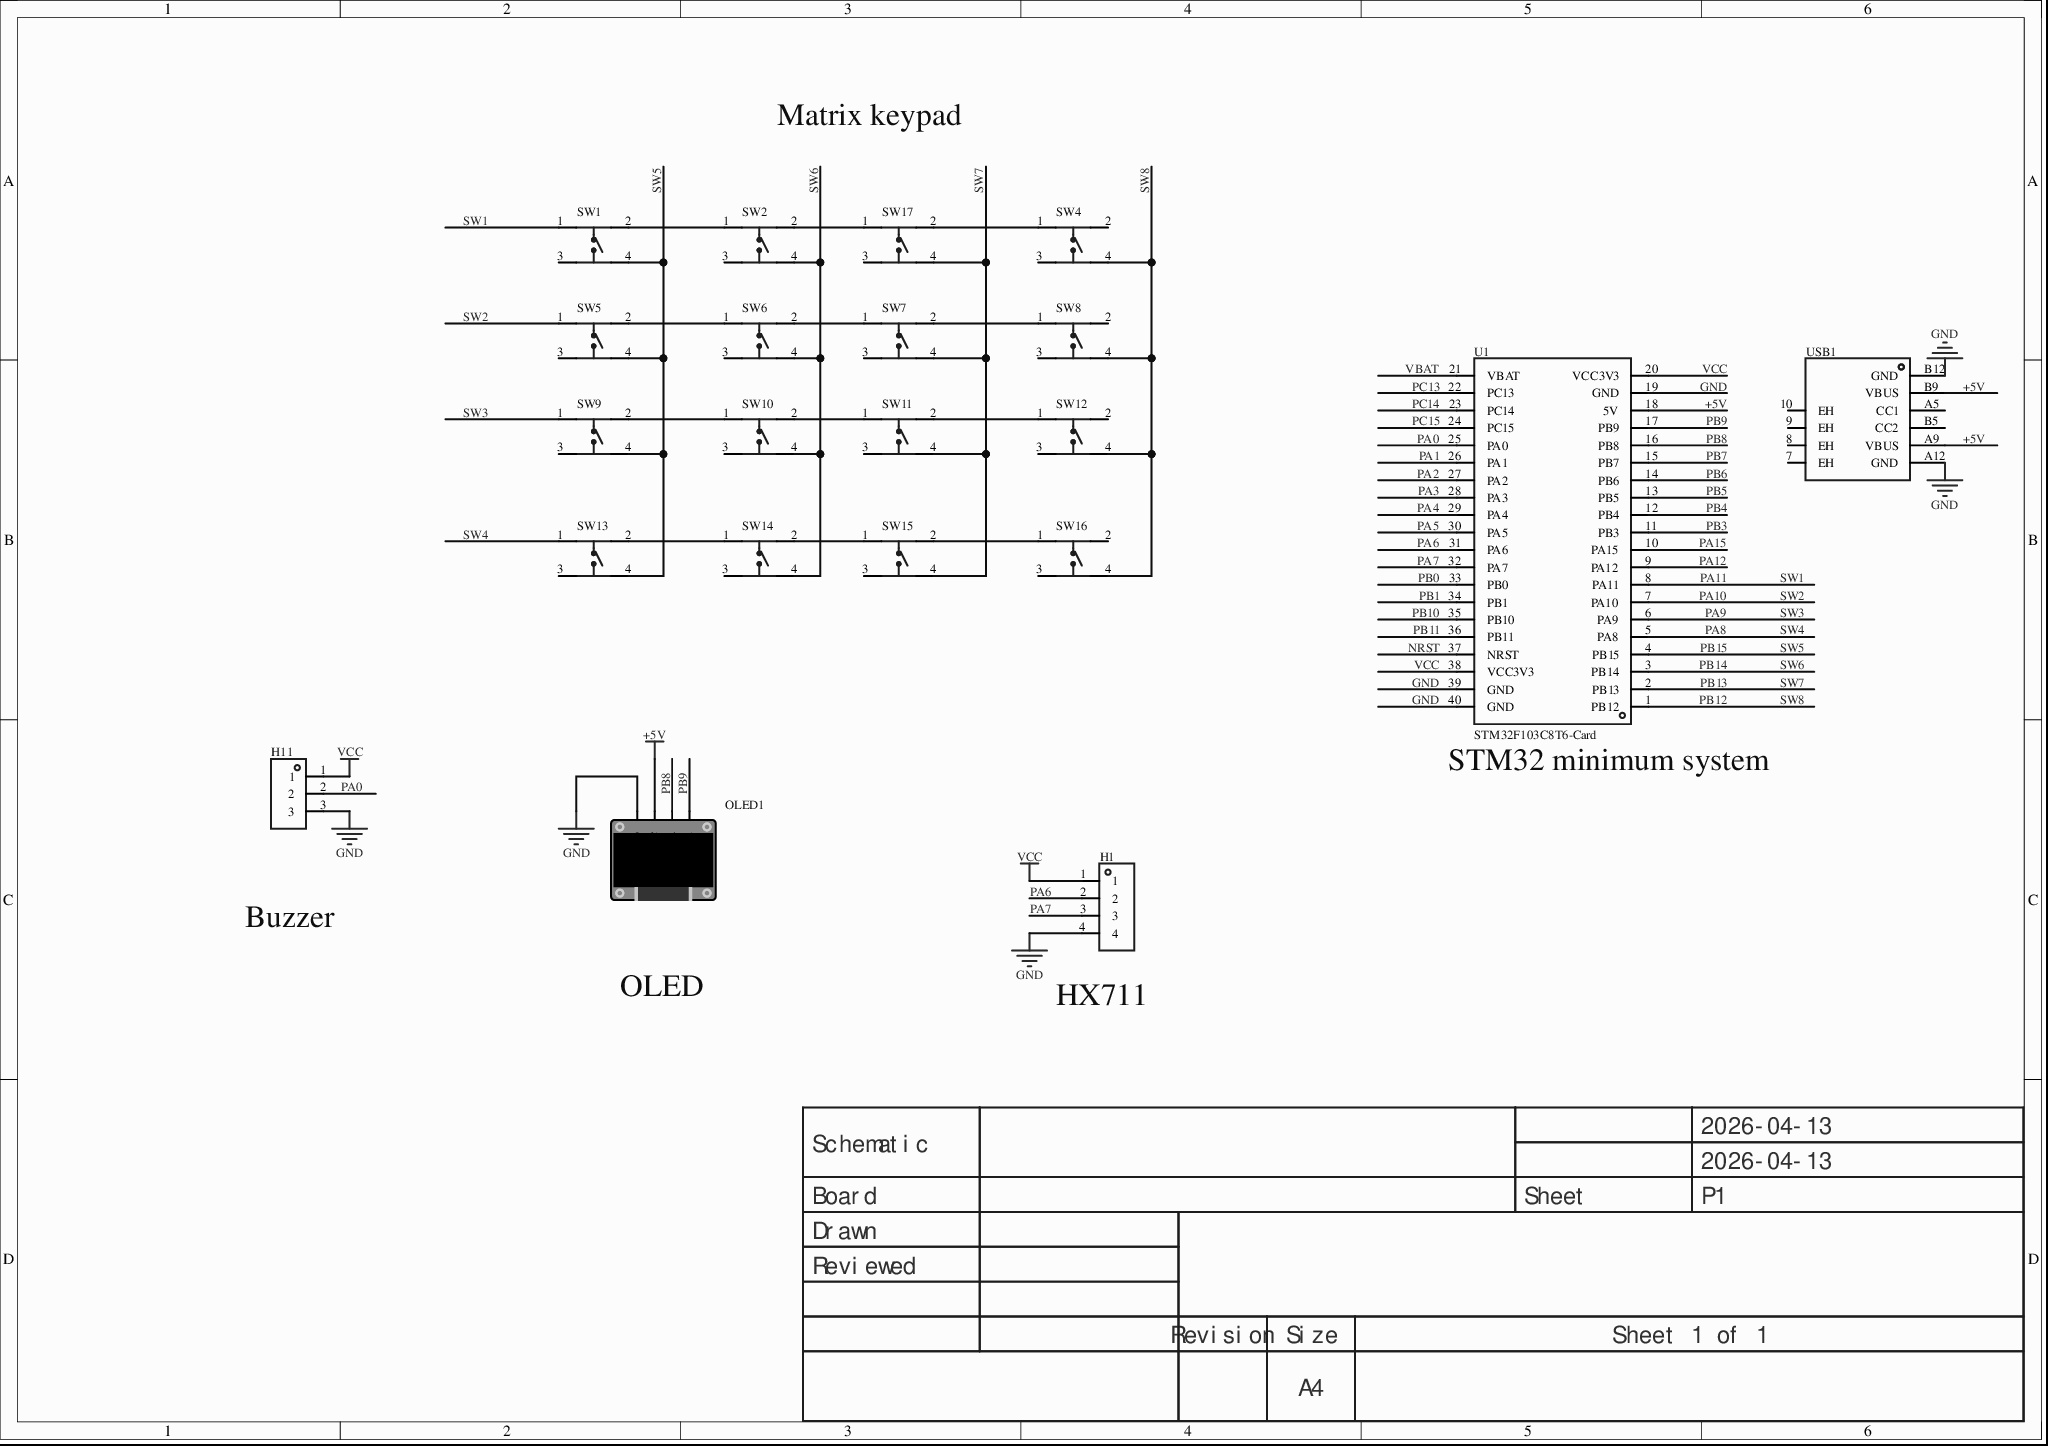
[diagram p0: MISC51803-3.schdoc]
# Altium project MISC51803-2.PrjPcb
1 sheet, 21 parts. Net scope: global (net labels, ports and power ports of the same name join across sheets).
Board file: MISC51803.pcbdoc

## Sheet MISC51803-3.schdoc
size 297 x 209 mm; Version: V1.0; @Project Name: MISC51803; @Update Date: 2026-04-13; @Create Date: 2026-04-13; @Board Name: MISC51803; @Create Time: 16:10:47; @Page Count: 1; @Page No: 1; @Schematic Name: MISC51803; @Update Time: 16:10:47; Size: A4

### Parts
H1  (no value)  [HDR-TH_4P-P2.54-V-M]
H11  (no value)  [HDR-TH_3P-P2.54-V-F]
OLED1  (no value)  [0.96OLED_4P]
SW1  KH-6X6X6H-TJ  [SW-TH_4P-L6.0-W6.0-P4.50-LS6.5]  (value not drawn)
SW2  KH-6X6X6H-TJ  [SW-TH_4P-L6.0-W6.0-P4.50-LS6.5]  (value not drawn)
SW4  KH-6X6X6H-TJ  [SW-TH_4P-L6.0-W6.0-P4.50-LS6.5]  (value not drawn)
SW5  KH-6X6X6H-TJ  [SW-TH_4P-L6.0-W6.0-P4.50-LS6.5]  (value not drawn)
SW6  KH-6X6X6H-TJ  [SW-TH_4P-L6.0-W6.0-P4.50-LS6.5]  (value not drawn)
SW7  KH-6X6X6H-TJ  [SW-TH_4P-L6.0-W6.0-P4.50-LS6.5]  (value not drawn)
SW8  KH-6X6X6H-TJ  [SW-TH_4P-L6.0-W6.0-P4.50-LS6.5]  (value not drawn)
SW9  KH-6X6X6H-TJ  [SW-TH_4P-L6.0-W6.0-P4.50-LS6.5]  (value not drawn)
SW10  KH-6X6X6H-TJ  [SW-TH_4P-L6.0-W6.0-P4.50-LS6.5]  (value not drawn)
SW11  KH-6X6X6H-TJ  [SW-TH_4P-L6.0-W6.0-P4.50-LS6.5]  (value not drawn)
SW12  KH-6X6X6H-TJ  [SW-TH_4P-L6.0-W6.0-P4.50-LS6.5]  (value not drawn)
SW13  KH-6X6X6H-TJ  [SW-TH_4P-L6.0-W6.0-P4.50-LS6.5]  (value not drawn)
SW14  KH-6X6X6H-TJ  [SW-TH_4P-L6.0-W6.0-P4.50-LS6.5]  (value not drawn)
SW15  KH-6X6X6H-TJ  [SW-TH_4P-L6.0-W6.0-P4.50-LS6.5]  (value not drawn)
SW16  KH-6X6X6H-TJ  [SW-TH_4P-L6.0-W6.0-P4.50-LS6.5]  (value not drawn)
SW17  KH-6X6X6H-TJ  [SW-TH_4P-L6.0-W6.0-P4.50-LS6.5]  (value not drawn)
U1  STM32F103C8T6-Card  [CONN-TH_L53.3-W22.9_STM32F103C8T6-CARD]
USB1  (no value)  [USB_ TYPE-C-6P]

### Nets
+5V: OLED1.2(VCC) U1.18(5V) USB1.A9(VBUS) USB1.B9(VBUS)
GND: H1.4 H11.3 OLED1.1(GND) U1.19(GND) U1.39(GND) U1.40(GND) USB1.A12(GND) USB1.B12(GND)
VCC: H1.1 H11.1 U1.20(VCC3V3) U1.38(VCC3V3)
NRST: U1.37(NRST)
PA0: H11.2 U1.25(PA0)
PA1: U1.26(PA1)
PA2: U1.27(PA2)
PA3: U1.28(PA3)
PA4: U1.29(PA4)
PA5: U1.30(PA5)
PA6: H1.2 U1.31(PA6)
PA7: H1.3 U1.32(PA7)
PA8: SW13.1 U1.5(PA8)  [also labelled SW4]
PA9: SW9.1 U1.6(PA9)  [also labelled SW3]
PA10: SW5.1 U1.7(PA10)  [also labelled SW2]
PA11: SW1.1 U1.8(PA11)  [also labelled SW1]
PA12: U1.9(PA12)
PA15: U1.10(PA15)
PB0: U1.33(PB0)
PB1: U1.34(PB1)
PB3: U1.11(PB3)
PB4: U1.12(PB4)
PB5: U1.13(PB5)
PB6: U1.14(PB6)
PB7: U1.15(PB7)
PB8: OLED1.3(SCL) U1.16(PB8)
PB9: OLED1.4(SDA) U1.17(PB9)
PB10: U1.35(PB10)
PB11: U1.36(PB11)
PB12: SW4.4 SW8.4 SW12.4 SW16.4 U1.1(PB12)  [also labelled SW8]
PB13: SW7.4 SW11.4 SW15.4 SW17.4 U1.2(PB13)  [also labelled SW7]
PB14: SW2.4 SW6.4 SW10.4 SW14.4 U1.3(PB14)  [also labelled SW6]
PB15: SW1.4 SW5.4 SW9.4 SW13.4 U1.4(PB15)  [also labelled SW5]
PC13: U1.22(PC13)
PC14: U1.23(PC14)
PC15: U1.24(PC15)
VBAT: U1.21(VBAT)
NetSW1_2: SW1.2 SW2.1
NetSW2_2: SW2.2 SW17.1
NetSW4_1: SW4.1 SW17.2
NetSW5_2: SW5.2 SW6.1
NetSW6_2: SW6.2 SW7.1
NetSW7_2: SW7.2 SW8.1
NetSW9_2: SW9.2 SW10.1
NetSW10_2: SW10.2 SW11.1
NetSW11_2: SW11.2 SW12.1
NetSW13_2: SW13.2 SW14.1
NetSW14_2: SW14.2 SW15.1
NetSW15_2: SW15.2 SW16.1

Not connected (* = marked no-connect by the designer): SW1 3*; SW2 3*; SW4 2* 3*; SW5 3*; SW6 3*; SW7 3*; SW8 2* 3*; SW9 3*; SW10 3*; SW11 3*; SW12 2* 3*; SW13 3*; SW14 3*; SW15 3*; SW16 2* 3*; SW17 3*; USB1 7(EH) 8(EH) 9(EH) 10(EH) A5(CC1) B5(CC2)

### Notes on the sheet
- Matrix keypad
- (near U1) STM32 minimum system
- Buzzer
- OLED
- (near H1) HX711
- 2026-04-13
- Schematic
- Board
- Sheet
- P1
- Drawn
- Reviewed
- Revision
- Size
- A4
- Sheet 1 of 1

### Library data of the parts
H1 = HDR-M_2.54_1x4P: Symbol: PZ254V-11-04P; ConvertToPcb: yes; ModelId: 112f4d05e8d64e99ab9a333894bea4f90819f05c4eef4c71ace90d822a990e87; ModelName: HDR-TH_4P-P2.54-M-LI-1X4P; ModelTransform: 399.999,104.7242,0,0,0,0,0,0,-118.11; Device: HDR-M_2.54_1x4P; AddInBom: yes; SupplierPart: C492403; Supplier Footprint: 插件; FootprintName: HDR-TH_4P-P2.54-V-M
H11 = HDR-F_2.54_1x3P: Symbol: PM254V-11-03-H85; 3D Model: f3b3cc5aae9641bf9e56fc160cef875b; 3D Model Transform: 299.9994,100,0,0,0,0,0,0,-118.11; ConvertToPcb: yes; ModelName: HDR2.54-F-LI-1X3P; Device: HDR-F_2.54_1x3P; Supplier Part: C541850; Supplier Footprint: 插件; AddInBom: yes; FootprintName: HDR-TH_3P-P2.54-V-F
OLED1 = 0.96OLED模块_4P: 3D Model: 79c000fdb68d45a296c2e9bedf4f9055; 3D Model Transform: 1393.69792,1318.895,0,0,0,0,0,-560.079,-137.795; ConvertToPcb: yes; Symbol: 0.96OLED模块_4P; Device: 0.96OLED模块_4P; Supplier Footprint: 插件; AddInBom: yes; FootprintName: 0.96OLED_4P; ModelName: 0.96OLED_4P
SW1 SW2 SW4-SW17 = KH-6X6X6H-TJ: Circuit structure: SPST; Button shape: round button; Actuating force: 2.6N; Mounting: through-hole; Switch length: 6mm; Switch width: 6mm; Switch height: 6mm; Bracket: none; Contact current: 50mA; Rated voltage: 12V; Operating life: -;; Manufacturer: kinghelm(金航标); 3D Model: 20eee248bc684ccd8cbdbb1d0d91ec6f; 3D Model Transform: 236.22,323.03,0,90,0,0,0,0,-137.795; with Bracket: No bracket; Actuator/Cap Color: Black; AddInBom: yes; ModelName: SW-TH_4P-L6.0-W6.0-H5.0-LS6.5-P4.50; Symbol: KH-6X6X6H-TJ; Device: KH-6X6X6H-TJ; LCSC Part Name: 6*6*6mm 直插 轻触开关; Supplier Part: C2837516; Manufacturer Part: KH-6X6X6H-TJ; Supplier Footprint: 插件-4P,6x6mm; JLCPCB Part Class: Extended library; Datasheet: https://item.szlcsc.com/datasheet/KH-6X6X6H-TJ/3009586.html; Supplier: LCSC; Circuit: SPST; Actuator Style: Round button; Operating Force: 2.6N; Mounting Type: Through-hole; Length: 6mm; Width: 6mm; Switch Height: 6mm; Contact Current: 50mA; Voltage Rating: 12V; Termination Style: PC pins; Life: -; Operating Temperature: -25℃~+70℃; ConvertToPcb: yes; FootprintName: SW-TH_4P-L6.0-W6.0-P4.50-LS6.5
U1 = STM32F103C8T6-Card: AddInBom: yes; Symbol: STM32F103C8T6-CARD; Device: STM32F103C8T6-Card; LCSC Part Name: STM32F103C8T6-Card; Supplier Part: C9900077949; Manufacturer Part: STM32F103C8T6-Card; Supplier Footprint: 插件; Supplier: LCSC; ConvertToPcb: yes; FootprintName: CONN-TH_L53.3-W22.9_STM32F103C8T6-CARD
USB1 = USB_ Type-C-6P: AddInBom: yes; ModelId: d4f492a4e6024845a13b3f6a4ef2d2cb0819f05c4eef4c71ace90d822a990e87; ModelName: USB-SMD_U262-061N-4BVC11; ModelTransform: 352.362,281.496,0,0,0,0,0,-47.244,-39.37; Symbol: USB_ TYPE-C-6P; Device: USB_ Type-C-6P; Supplier Footprint: SMD; ConvertToPcb: yes; FootprintName: USB_ TYPE-C-6P